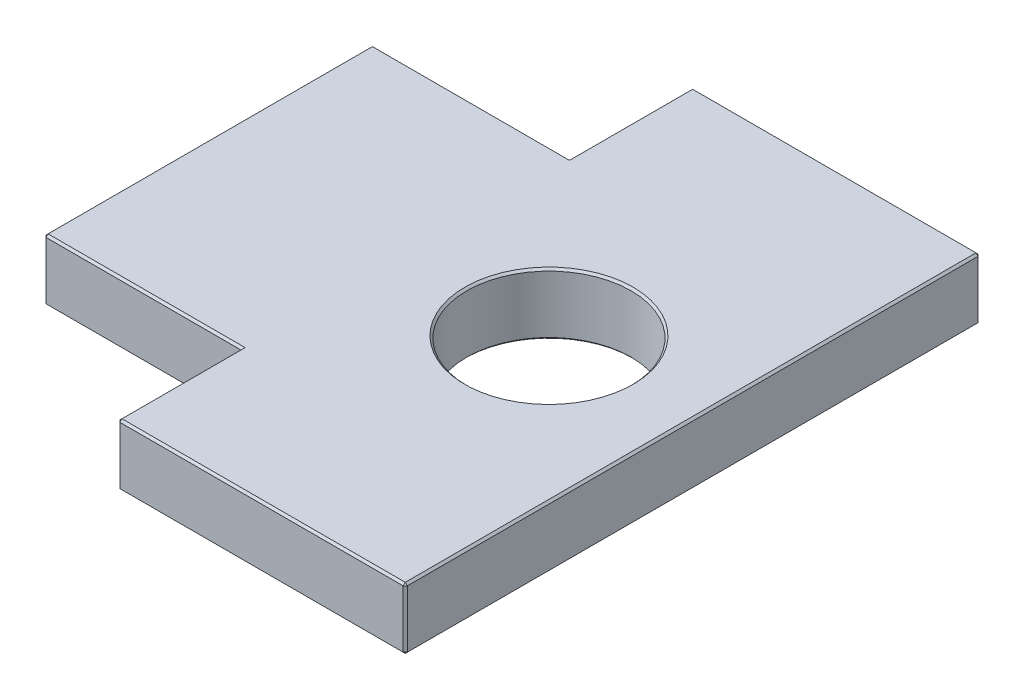
from build123d import *

# Parameters (mm, degrees)
SKETCH_1_R      = 20
EXTRUDE_1_DEPTH = 15
CHAMFER_1_SIZE  = 0.5


with BuildPart() as part:
    # 草图1 → 凸台-拉伸1 (new body)
    with BuildSketch(Plane(origin=(0, 0, 0), x_dir=(1, 0, 0), z_dir=(0, 1, 0))):
        Polygon((0, 70), (0, -70), (-70, -70), (-70, -40), (-118, -40), (-118, 40), (-70, 40), (-70, 70), align=None)
        with Locations(Location((-35, 0, 0), (0, 0, 270))):
            Circle(SKETCH_1_R, mode=Mode.SUBTRACT)
    extrude(amount=EXTRUDE_1_DEPTH)

    # 倒角1
    chamfer_1_edges = [part.edges().sort_by_distance(p)[0] for p in [
        (-35, 15, -70),
        (0, 0, 0),
        (-35, 0, 70),
        (-70, 15, -55),
        (-70, 7.5, 70),
        (-118, 7.5, 40),
        (-118, 7.5, -40),
        (-70, 7.5, -70),
        (0, 7.5, -70),
        (0, 7.5, 70),
        (-94, 15, -40),
        (-118, 15, 0),
        (-35, 0, -20),
        (-35, 15, -20),
        (-94, 15, 40),
        (-70, 15, 55),
        (-35, 15, 70),
        (0, 15, 0),
        (-70, 0, 55),
        (-94, 0, 40),
        (-118, 0, 0),
        (-94, 0, -40),
        (-70, 0, -55),
        (-35, 0, -70),
    ]]
    chamfer(chamfer_1_edges, length=CHAMFER_1_SIZE)


solid = part.part
